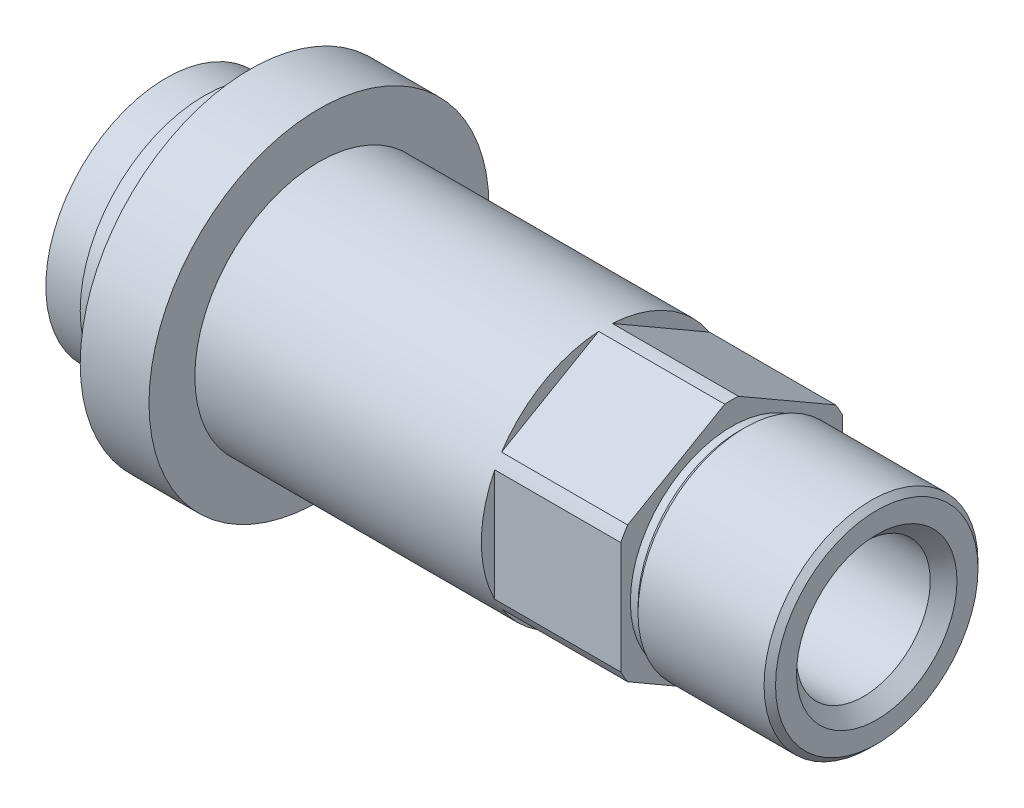
from build123d import *

# Parameters (mm, degrees)
CHAMFER1_SIZE      = 1.5
CUT_EXTRUDE1_START = -33
CUT_EXTRUDE1_DEPTH = 71
CIRPATTERN1_COUNT  = 6
CHAMFER3_SIZE      = 3.5


with BuildPart() as part:
    # Sketch1 → Revolve1 (revolve)
    with BuildSketch(Plane.XY, mode=Mode.PRIVATE) as revolve1_sk:
        Polygon((-34.5, 28), (-36, 26.5), (-38, 26.5), (-38, 28), (-38, 32.5), (-146, 32.5), (-146, 44.5), (-164, 44.5), (-164, 32.5), (-176, 32.5), (-176, 31.5), (-186, 31.5), (-186, 0), (-176, 0), (-164, 0), (-146, 0), (-38, 0), (0, 0), (0, 28), align=None)
    revolve(revolve1_sk.sketch.rotate(Axis((0, 0, 0), (-1, 0, 0)), 90), axis=Axis((0, 0, 0), (-1, 0, 0)))

    # Chamfer1
    chamfer1_edges = [part.edges().sort_by_distance(p)[0] for p in [
        (0, 0, 28),
    ]]
    chamfer(chamfer1_edges, length=CHAMFER1_SIZE)

    # Sketch2 → Cut-Extrude1 (cut)
    with BuildSketch(Plane(origin=(-38, 0, 0), x_dir=(0, 0, -1), z_dir=(1, 0, 0)).offset(CUT_EXTRUDE1_START)):
        with BuildLine():
            Line((1.79419424, 32.450437085), (27.20580576, 17.779036334))
            ThreePointArc((27.20580576, 17.779036334), (16.25, 28.145825623), (1.79419424, 32.450437085))
        make_face()
    cut_extrude1 = extrude(amount=CUT_EXTRUDE1_DEPTH, mode=Mode.SUBTRACT)

    # CirPattern1: Cut-Extrude1 ×6 about axis
    cirpattern1_axis = Axis((0, 0, 0), (1, 0, 0))
    for i in range(1, CIRPATTERN1_COUNT):
        add(cut_extrude1.rotate(cirpattern1_axis, i * 360 / CIRPATTERN1_COUNT), mode=Mode.SUBTRACT)

    # Sketch4 → Cut-Revolve2 (revolve, cut)
    with BuildSketch(Plane.XY):
        Polygon((0, 0), (-70, 0), (-186, 0), (-186, 21), (-70, 21), (-66.5, 17.5), (0, 17.5), align=None)
    revolve(axis=Axis((0, 0, 0), (-1, 0, 0)), mode=Mode.SUBTRACT)

    # Chamfer3
    chamfer3_edges = [part.edges().sort_by_distance(p)[0] for p in [
        (0, -17.5, 0),
    ]]
    chamfer(chamfer3_edges, length=CHAMFER3_SIZE)


solid = part.part
